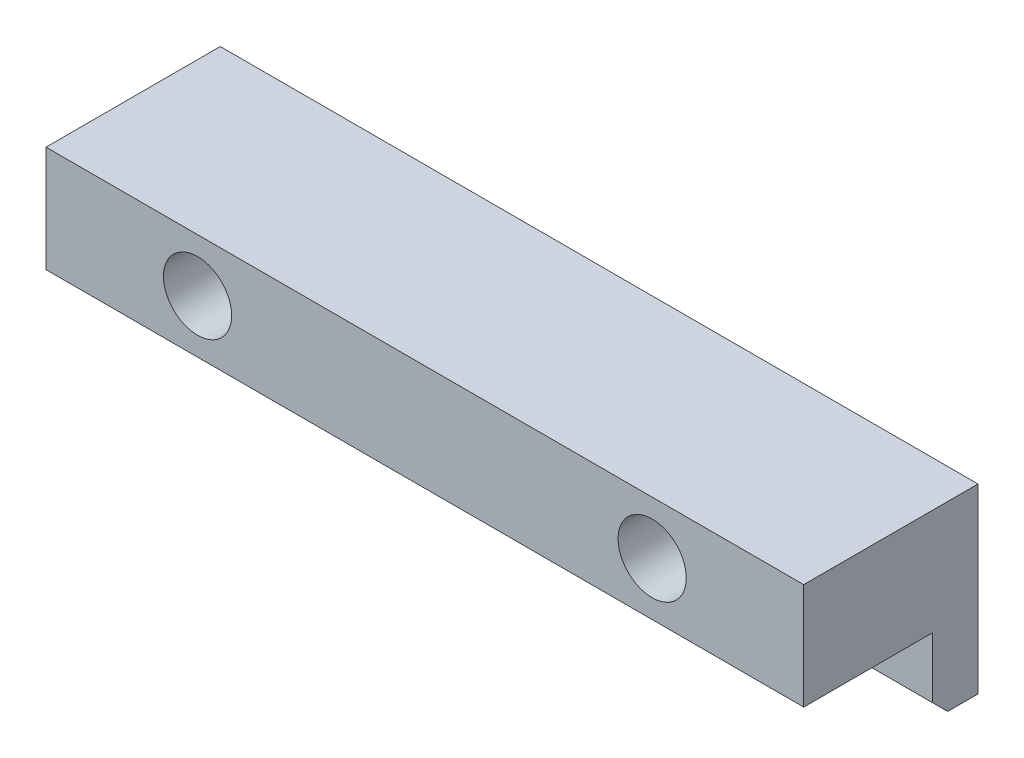
SolidWorks part; units mm, degrees
ref_plane "Front Plane" through (0, 0, 0) normal (0, 0, 1) x (1, 0, 0)
ref_plane "Top Plane" through (0, 0, 0) normal (0, 1, 0) x (1, 0, 0)
ref_plane "Right Plane" through (0, 0, 0) normal (1, 0, 0) x (0, 0, -1)
other "Configuration Table"
sketch "Sketch1" plane through (0, 0, 0) normal (0, 0, 1) x (1, 0, 0)
  line L1 (0, 0) -> (50, 0)
  line L2 (0, 0) -> (0, 12)
  line L3 (0, 12) -> (50, 12)
  line L4 (50, 0) -> (50, 12)
  dimension "D1" = 50
  dimension "D2" = 12
extrude "Boss-Extrude1" add sketch "Sketch1" along normal blind 5
sketch "Sketch2" plane through (0, 0, 5) normal (0, 0, 1) x (1, 0, 0)
  line L0 (25, 12) -> (25, -1.9406) construction
  line L1 (50, 12) -> (0, 12) construction
  circle A0 centre (10, 8.5) radius 2.25
  circle A1 centre (40, 8.5) radius 2.25
  dimension "D1" = 4.5
  dimension "D4" = 4.5
  dimension "D2" = 15
  dimension "D3" = 15
  dimension "D5" = 3.5
  dimension "D6" = 3.5
extrude "Cut-Extrude1" cut sketch "Sketch2" against normal through all
sketch "Sketch3" plane through (50, 0, 0) normal (1, 0, 0) x (0, 0, -1)
  line L1 (-5, 0) -> (-3, 0)
  line L2 (-5, 0) -> (-5, 5)
  line L3 (-5, 5) -> (-3, 5)
  line L4 (-3, 0) -> (-3, 5)
  dimension "D1" = 2
  dimension "D2" = 5
extrude "Cut-Extrude2" cut sketch "Sketch3" against normal through all
chamfer "Chamfer1" distance 1 angle 45 1 edges at (25, 0, 3)
other "Move Face1" face at (12.25, 8.5, 5) parameters "D1"=6.5
